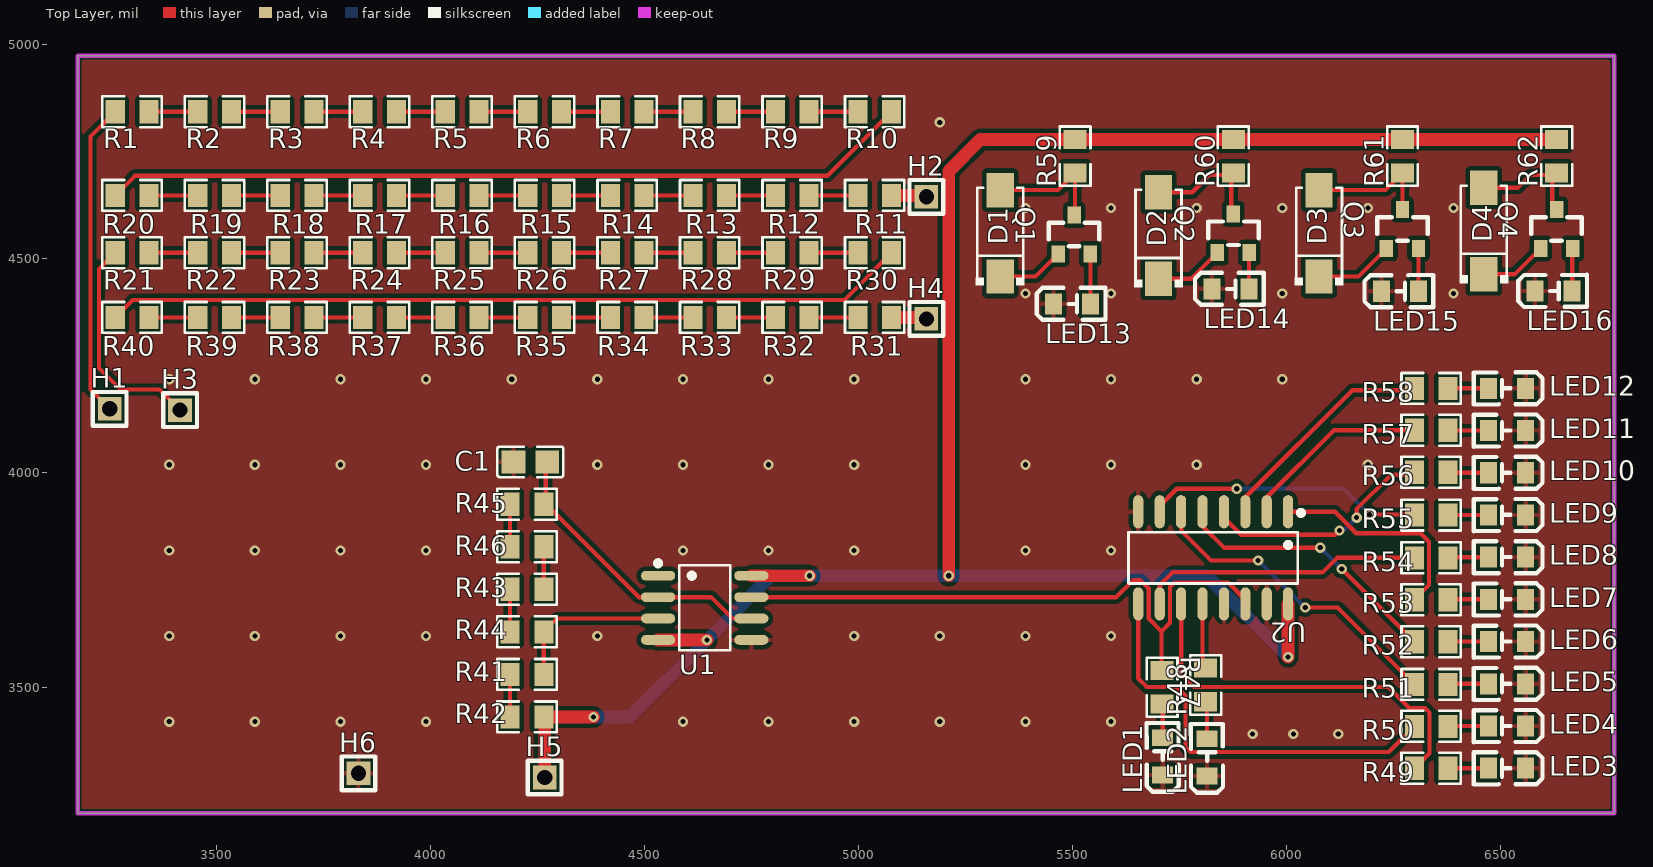
[diagram p0: Top Layer view]
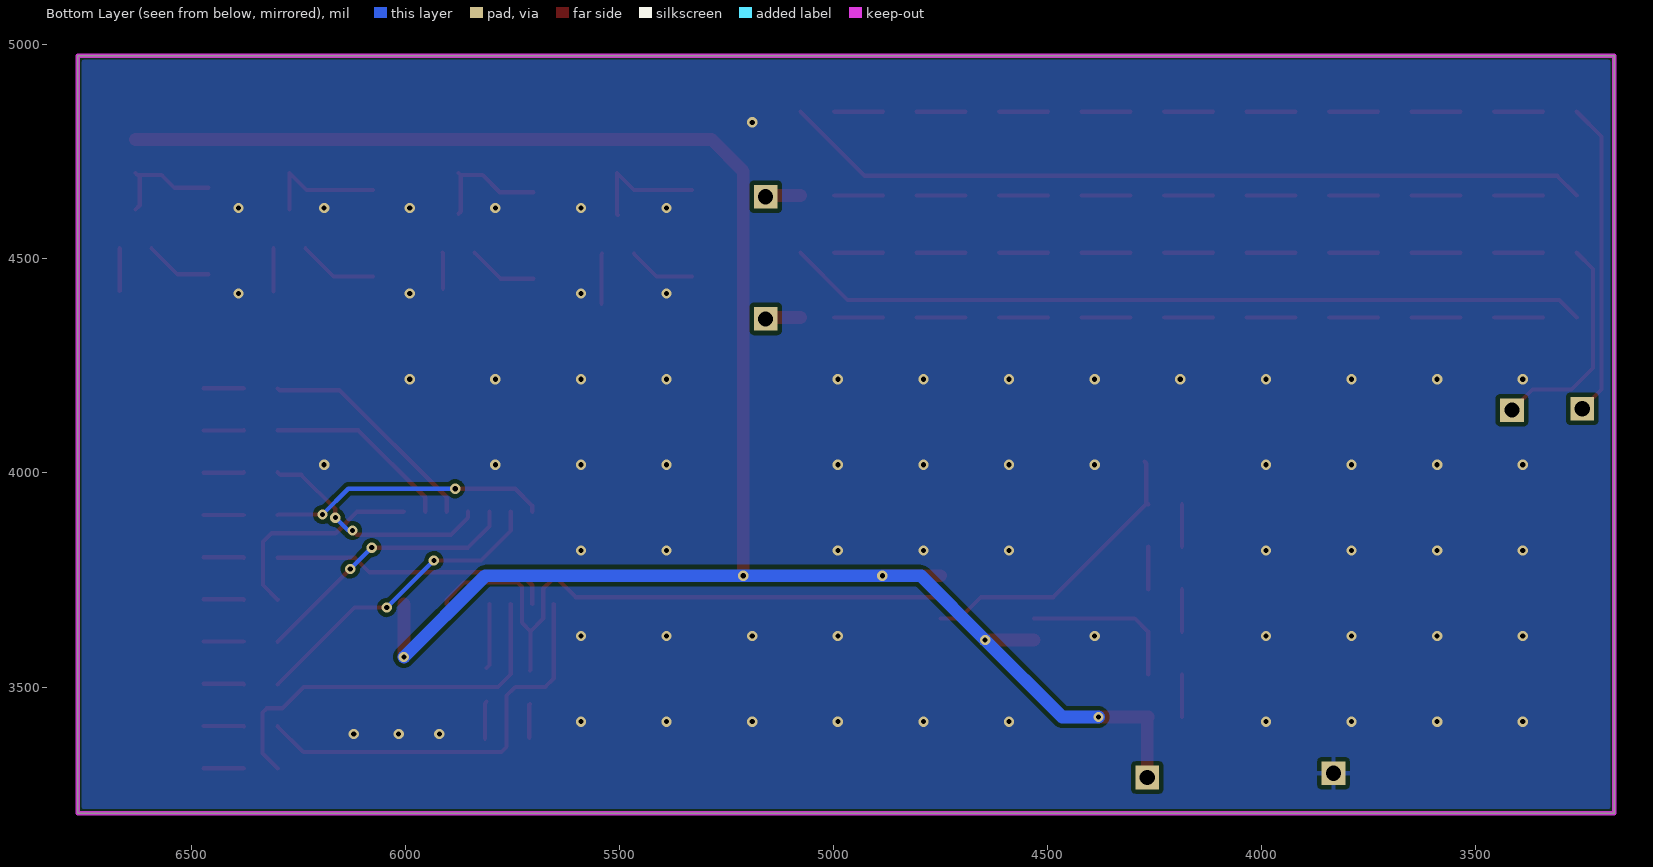
[diagram p1: Bottom Layer view, seen from below]
# Altium PCB MISC75384.pcbdoc
Units mil, origin at the board's own origin, x right, y up, seen from the top; angles counter-clockwise.
Board outline 3590 x 1770 mil, 2 copper layers (Top Layer, Bottom Layer), stack 62.206 mil thick; 95 components, 86 nets, 208 pads, 80 vias.

## Layer stack, top to bottom
Top Solder Mask Layer: solder mask 0.394, Dk 3.3
Top Layer: signal copper 1.379
Dielectric1: surface 59.449, FR4, Dk 4.5
Bottom Layer: signal copper 1.378
Bottom Solder Mask Layer: solder mask 0.394, Dk 3.3

## Board outline
3175,4975 3175,3205 6765,3205 6765,4975

## Design rules (kind name [scope] priority, off if disabled: settings)
BoardOutlineClearance copperThickness2oz_1 [All] p2 off: genericclearance=7.99 ignorepadtopadclearanceinfootprint=FALSE except(0: Arc-SplitContinuation Track-SplitContinuation SMDPad-SplitContinuation THPad-SplitContinuation Via-SplitContinuation Fill-SplitContinuation Region-SplitContinuation Poly-SplitContinuation Text-SplitContinuation Hole-SplitContinuation; 5.98: Arc-CutoutEdge SMDPad-CutoutEdge THPad-CutoutEdge Via-CutoutEdge Fill-CutoutEdge Region-CutoutEdge Text-CutoutEdge; 6.93: Hole-OutlineEdge Hole-CutoutEdge; 10: Poly-OutlineEdge Poly-CutoutEdge; 11.81: Arc-OutlineEdge Track-OutlineEdge SMDPad-OutlineEdge THPad-OutlineEdge Via-OutlineEdge Fill-OutlineEdge Region-OutlineEdge Text-OutlineEdge Track-CutoutEdge)
BoardOutlineClearance copperThickness1oz_1 [All] p4: genericclearance=4.02 ignorepadtopadclearanceinfootprint=FALSE except(0: Arc-SplitContinuation Track-SplitContinuation SMDPad-SplitContinuation THPad-SplitContinuation Via-SplitContinuation Fill-SplitContinuation Region-SplitContinuation Poly-SplitContinuation Text-SplitContinuation Hole-SplitContinuation; 6: SMDPad-CutoutEdge THPad-CutoutEdge Via-CutoutEdge Fill-CutoutEdge Region-CutoutEdge Text-CutoutEdge; 6.93: Hole-OutlineEdge Hole-CutoutEdge; 10: Poly-OutlineEdge Poly-CutoutEdge; 11.8: Arc-OutlineEdge Track-OutlineEdge SMDPad-OutlineEdge THPad-OutlineEdge Via-OutlineEdge Fill-OutlineEdge Region-OutlineEdge Text-OutlineEdge; 11.81: Arc-CutoutEdge Track-CutoutEdge)
Clearance copperThickness2oz [All] p1 off: gap=7.99 ignorepadtopadclearanceinfootprint=FALSE except(5.98: SMDPad-Track SMDPad-SMDPad THPad-Track SMDPad-THPad THPad-THPad Track-Via SMDPad-Via THPad-Via Via-Via Fill-Track Region-Track Fill-SMDPad Region-SMDPad Fill-THPad Region-THPad Fill-Via Region-Via Fill-Fill Fill-Region Region-Region Arc-Track Arc-SMDPad Arc-THPad Arc-Via Fill-Arc Region-Arc Arc-Arc Text-Track SMDPad-Text Text-THPad Text-Via Fill-Text Region-Text Arc-Text Text-Text; 6.93: Hole-Track Hole-SMDPad Hole-THPad Hole-Via Fill-Hole Region-Hole Hole-Arc Hole-Text; 10: Poly-Track Poly-SMDPad Poly-THPad Poly-Via Poly-Fill Poly-Region Poly-Poly Poly-Arc Poly-Text Poly-Hole)
Clearance copperThickness1oz [All] p3: gap=4.02 ignorepadtopadclearanceinfootprint=FALSE except(5.98: SMDPad-Track SMDPad-SMDPad THPad-Track SMDPad-THPad THPad-THPad Track-Via SMDPad-Via THPad-Via Via-Via Fill-Track Region-Track Fill-SMDPad Region-SMDPad Fill-THPad Region-THPad Fill-Via Region-Via Fill-Fill Fill-Region Region-Region; 6: Arc-Track Arc-SMDPad Arc-THPad Arc-Via Fill-Arc Region-Arc Arc-Arc Text-Track SMDPad-Text Text-THPad Text-Via Fill-Text Region-Text Arc-Text Text-Text; 6.93: Hole-Track Hole-SMDPad Hole-THPad Hole-Via Fill-Hole Region-Hole Hole-Arc Hole-Text; 10: Poly-Track Poly-SMDPad Poly-THPad Poly-Via Poly-Fill Poly-Region Poly-Poly Poly-Arc Poly-Text Poly-Hole)
Creepage creepage [All] p1: checkdistance=0 ignoreinternallayers=TRUE applytopolygonpour=TRUE
DiffPairsRouting differentialPair [All] p1: maxlimit=6 minlimit=6 mostfreqgap=6 toplayer_minwidth=5 toplayer_prefwidth=10 toplayer_maxwidth=100 toplayer_mingap=6 toplayer_prefgap=6 toplayer_maxgap=6 bottomlayer_minwidth=5 bottomlayer_prefwidth=10 bottomlayer_maxwidth=100 bottomlayer_mingap=6 bottomlayer_prefgap=6 bottomlayer_maxgap=6 maxuncoupledlength=10
HoleToHoleClearance otherClearance [All] p1: gap=11.81 allowstackedmicrovias=TRUE
Length netLength [All] p1: minlimit=0 maxlimit=0
MatchedLengths netLengthTolerance [All] p1: tolerance=1000
PasteMaskExpansion pasteMaskExpansion [All] p1: expansion=0
PlaneConnect innerPlane [All] p1: planeconnectstyle=Relief reliefexpansion=20 reliefentries=4 reliefconductorwidth=10 reliefairgap=10
PolygonConnect copperRegion [(InNet('GND') OR InNet('$1N69'))] p1: connectstyle=Relief reliefconductorwidth=10 reliefentries=4 polygonreliefangle="90 Angle" airgapwidth=10 via.connectstyle=Relief via.reliefconductorwidth=10 via.reliefentries=4 via.polygonreliefangle="90 Angle" via.airgapwidth=10
RoutingVias viaSize [All] p1: holewidth=12.01 width=24.02 viastyle="Through Hole" minholewidth=11.81 minwidth=19.68 maxholewidth=248.03 maxwidth=393.7
SolderMaskExpansion solderMaskExpansion [IsVia] p1: expansion=-1000 istentingtop=TRUE
SolderMaskExpansion solderMaskExpansion [All] p2: expansion=2 istentingtop=FALSE
Width copperThickness2oz_2 [All] p1 off: maxlimit=100 minlimit=8 preferedwidth=10
Width copperThickness1oz_2 [All] p2: maxlimit=100 minlimit=5 preferedwidth=10

## Components (designator, comment, footprint, x,y, rotation, side; value= is the part's Value field where it differs from the comment)
C1 "100nF" C0805 4232.64,4025.93 r0 top
D1 "" SMA_1N4007 5330,4560 r90 top
D2 "" SMA_1N4007 5700,4555 r90 top
D3 "" SMA_1N4007 6075,4560 r90 top
D4 "" SMA_1N4007 6460,4565 r90 top
H1 "" HDR-TH_1P-V-M_XKB_X4611WV-01I-C28D40 3250,4150 r0 top
H2 "" HDR-TH_1P-V-M_XKB_X4611WV-01I-C28D40 5157.69,4645.25 r0 top
H3 "" HDR-TH_1P-V-M_XKB_X4611WV-01I-C28D40 3414.27,4146.83 r0 top
H4 "" HDR-TH_1P-V-M_XKB_X4611WV-01I-C28D40 5157.69,4359.98 r0 top
H5 "" HDR-TH_1P-V-M_XKB_X4611WV-01I-C28D40 4266.12,3288.68 r0 top
H6 "" HDR-TH_1P-V-M_XKB_X4611WV-01I-C28D40 3831.12,3298.4 r0 top
LED1 "" LED_0805 5710,3340 r90 top
LED2 "" LED_0805 5813.62,3337.66 r90 top
LED3 "" LED_0805 6512.42,3310.52 r180 top
LED4 "" LED_0805 6512.42,3409.12 r180 top
LED5 "" LED_0805 6512.42,3507.72 r180 top
LED6 "" LED_0805 6512.42,3606.31 r180 top
LED7 "" LED_0805 6512.42,3704.91 r180 top
LED8 "" LED_0805 6512.42,3803.51 r180 top
LED9 "" LED_0805 6512.42,3902.11 r180 top
LED10 "" LED_0805 6512.42,4000.71 r180 top
LED11 "" LED_0805 6512.42,4099.3 r180 top
LED12 "" LED_0805 6512.42,4197.9 r180 top
LED13 "" LED_0805 5500,4395 r0 top
LED14 "" LED_0805 5870,4430 r0 top
LED15 "" LED_0805 6266.02,4424.29 r0 top
LED16 "" LED_0805 6625,4425 r0 top
Q1 "" S8050_SOT-23 5502.85,4557.14 r270 top
Q2 "" S8050_SOT-23 5875,4560 r270 top
Q3 "" S8050_SOT-23 6270,4570 r270 top
Q4 "" S8050_SOT-23 6630,4570 r270 top
R1 "10K" R0805 3302.34,4844.04 r0 top
R2 "10K" R0805 3495.07,4844.04 r0 top
R3 "10K" R0805 3687.81,4844.04 r0 top
R4 "10K" R0805 3880.54,4844.04 r0 top
R5 "10K" R0805 4073.28,4844.04 r0 top
R6 "10K" R0805 4266.01,4844.04 r0 top
R7 "10K" R0805 4458.75,4844.04 r0 top
R8 "10K" R0805 4651.48,4844.04 r0 top
R9 "10K" R0805 4844.22,4844.04 r0 top
R10 "10K" R0805 5036.95,4844.04 r0 top
R11 "10K" R0805 5036.95,4648.25 r180 top
R12 "10K" R0805 4844.22,4648.25 r180 top
R13 "10K" R0805 4651.48,4648.25 r180 top
R14 "10K" R0805 4458.75,4648.25 r180 top
R15 "10K" R0805 4266.01,4648.25 r180 top
R16 "10K" R0805 4073.28,4648.25 r180 top
R17 "10K" R0805 3880.54,4648.25 r180 top
R18 "10K" R0805 3687.81,4648.25 r180 top
R19 "10K" R0805 3495.07,4648.25 r180 top
R20 "10K" R0805 3302.34,4648.25 r180 top
R21 "15K" R0805 3302.34,4514.29 r0 top
R22 "15K" R0805 3495.07,4514.29 r0 top
R23 "15K" R0805 3687.81,4514.29 r0 top
R24 "15K" R0805 3880.54,4514.29 r0 top
R25 "15K" R0805 4073.28,4514.29 r0 top
R26 "15K" R0805 4266.01,4514.29 r0 top
R27 "15K" R0805 4458.75,4514.29 r0 top
R28 "15K" R0805 4651.48,4514.29 r0 top
R29 "15K" R0805 4844.22,4514.29 r0 top
R30 "15K" R0805 5036.95,4514.29 r0 top
R31 "15K" R0805 5036.95,4363.3 r180 top
R32 "15K" R0805 4844.22,4363.3 r180 top
R33 "15K" R0805 4651.48,4363.3 r180 top
R34 "15K" R0805 4458.75,4363.3 r180 top
R35 "15K" R0805 4266.01,4363.3 r180 top
R36 "15K" R0805 4073.28,4363.3 r180 top
R37 "15K" R0805 3880.54,4363.3 r180 top
R38 "15K" R0805 3687.81,4363.3 r180 top
R39 "15K" R0805 3495.07,4363.3 r180 top
R40 "15K" R0805 3302.34,4363.3 r180 top
R41 "10K" R0805 4224.66,3529.41 r0 top
R42 "10K" R0805 4224.66,3430 r180 top
R43 "10K" R0805 4224.66,3728.23 r0 top
R44 "10K" R0805 4224.66,3628.82 r180 top
R45 "10K" R0805 4224.66,3927.05 r0 top
R46 "10K" R0805 4224.66,3827.64 r180 top
R47 "1K" R0805 5708.24,3499.45 r270 top
R48 "1K" R0805 5810,3505 r90 top
R49 "10K" R0805 6337.09,3310.12 r0 top
R50 "10K" R0805 6337.09,3408.02 r0 top
R51 "10K" R0805 6337.09,3505.92 r0 top
R52 "10K" R0805 6337.09,3605.92 r0 top
R53 "10K" R0805 6337.09,3703.82 r0 top
R54 "10K" R0805 6337.09,3801.71 r0 top
R55 "10K" R0805 6337.09,3901.71 r0 top
R56 "10K" R0805 6337.09,4001.71 r0 top
R57 "10K" R0805 6337.09,4099.61 r0 top
R58 "10K" R0805 6337.09,4197.51 r0 top
R59 "1K" R0805 5505,4740 r90 top
R60 "1K" R0805 5875,4740 r90 top
R61 "1K" R0805 6270,4740 r90 top
R62 "1K" R0805 6630,4740 r90 top
U1 "NE555" SOP-8_L5.0-W4.0-P1.27-LS6.0-BL 4640,3685 r270 top
U2 "CD4017BM96G4" SOIC-16_L9.9-W3.9-P1.27-LS6.0-BL 5827.85,3801.71 r180 top

## Footprints (in the part's own frame and the unit in brackets; to place one, negate y for a bottom-side part, rotate by r counter-clockwise, add the part's x,y. Pads: shape width x height; smd on the part's side, far side on the other; paste and mask are expansions set on the pad)
C0805 [mm]
  rect 1.41x1.35 smd paste-100 mask+0.051: 1(-1,0) 2(1,0)
  silkscreen extent -1.96,-0.9 1.96,0.9
HDR-TH_1P-V-M_XKB_X4611WV-01I-C28D40 [mm]
  rect 1.4x1.4 hole 0.9: 1(0,0)
  silkscreen extent -1,-1 1,1
LED_0805 [mm]
  rect 1x1.25 smd paste+0 mask+0.051: 1(-1.15,0.005) 2(1.05,0.005)
  silkscreen extent -2.15,-0.94 1.93,0.97
R0805 [mm]
  rect 1.133x1.377 smd paste-100 mask+0.051: 1(-1,0) 2(1,0)
  silkscreen extent -1.76,-0.92 1.76,0.92
S8050_SOT-23 [mm]
  rect 1x0.8 smd paste+0 mask+0.051: 1(1.15,-0.95) 2(1.15,0.95) 3(-1.15,0)
  silkscreen extent -0.7,-1.5 0.7,1.5
SMA_1N4007 [mil]
  rect 80.57x63.78 smd paste+0 mask+2: 1(-101,0) 2(101,0)
  silkscreen extent -121,-57 106,57
SOIC-16_L9.9-W3.9-P1.27-LS6.0-BL [mil]
  oval 23.7x77.6 smd: 1(-175,-107.7) 2(-125,-107.7) 3(-75,-107.7) 4(-25,-107.7) 5(25,-107.7) 6(75,-107.7) 7(125,-107.7) 8(175,-107.7) 9(175,107.7) 10(125,107.7) 11(75,107.7) 12(25,107.7) 13(-25,107.7) 14(-75,107.7) 15(-125,107.7) 16(-175,107.7)
  silkscreen extent -211,-111 198,60
SOP-8_L5.0-W4.0-P1.27-LS6.0-BL [mil]
  oval 22.6x80.14 smd: 1(-75,-108.97) 2(-25,-108.97) 3(25,-108.97) 4(75,-108.97) 5(75,108.97) 6(25,108.97) 7(-25,108.97) 8(-75,108.97)
  silkscreen extent -110,-115 99,60

## Via types
v1: diameter 24.02, hole 12, Top Layer to Bottom Layer, 80 vias

## Nets (pads, with @x,y where several pads share a name; then routed paths per layer and width w, separated by ;. In a path a pad name is that pad's centre, name@x,y a point inside that pad or via, vN(x,y) a via of type N, cw(c..) or ccw(c..) an arc to the next point about the centre after c; other vN are vias at no path point)
$1N1: R1.2 R2.1 | length 114
  Top Layer w10: R1.2 R2.1
$1N2: R2.2 R3.1 | length 114
  Top Layer w10: R2.2 R3.1
$1N3: R3.2 R4.1 | length 114
  Top Layer w10: R3.2 R4.1
$1N4: R4.2 R5.1 | length 114
  Top Layer w10: R4.2 R5.1
$1N5: R5.2 R6.1 | length 114
  Top Layer w10: R5.2 R6.1
$1N6: R7.2 R8.1 | length 114
  Top Layer w10: R7.2 R8.1
$1N7: R6.2 R7.1 | length 114
  Top Layer w10: R6.2 R7.1
$1N8: R9.2 R10.1 | length 114
  Top Layer w10: R9.2 R10.1
$1N9: R8.2 R9.1 | length 114
  Top Layer w10: R8.2 R9.1
$1N10: R18.2 R19.1 | length 114
  Top Layer w10: R19.1 R18.2
$1N11: R16.2 R17.1 | length 114
  Top Layer w10: R17.1 R16.2
$1N12: R17.2 R18.1 | length 114
  Top Layer w10: R18.1 R17.2
$1N13: R19.2 R20.1 | length 114
  Top Layer w10: R20.1 R19.2
$1N14: R15.2 R16.1 | length 114
  Top Layer w10: R16.1 R15.2
$1N15: R14.2 R15.1 | length 114
  Top Layer w10: R15.1 R14.2
$1N16: R13.2 R14.1 | length 114
  Top Layer w10: R14.1 R13.2
$1N17: R12.2 R13.1 | length 114
  Top Layer w10: R13.1 R12.2
$1N18: R11.2 R12.1 | length 114
  Top Layer w10: R12.1 R11.2
$1N19: R10.2 R20.2 | length 1894.5
  Top Layer w10: R20.2 3308.76,4694.04 4926.32,4694.04 R10.2
$1N24: R30.2 R40.2 | length 1875.9
  Top Layer w10: R40.2 3303.96,4404.3 4966.32,4404.3 R30.2
$1N25: R28.2 R29.1 | length 114
  Top Layer w10: R28.2 R29.1
$1N26: R38.2 R39.1 | length 114
  Top Layer w10: R39.1 R38.2
$1N27: R26.2 R27.1 | length 114
  Top Layer w10: R26.2 R27.1
$1N28: R36.2 R37.1 | length 114
  Top Layer w10: R37.1 R36.2
$1N29: R27.2 R28.1 | length 114
  Top Layer w10: R27.2 R28.1
$1N30: R39.2 R40.1 | length 114
  Top Layer w10: R40.1 R39.2
$1N31: R29.2 R30.1 | length 114
  Top Layer w10: R29.2 R30.1
$1N32: R37.2 R38.1 | length 114
  Top Layer w10: R38.1 R37.2
$1N33: R25.2 R26.1 | length 114
  Top Layer w10: R25.2 R26.1
$1N34: R35.2 R36.1 | length 114
  Top Layer w10: R36.1 R35.2
$1N35: R24.2 R25.1 | length 114
  Top Layer w10: R24.2 R25.1
$1N36: R34.2 R35.1 | length 114
  Top Layer w10: R35.1 R34.2
$1N37: R23.2 R24.1 | length 114
  Top Layer w10: R23.2 R24.1
$1N38: R33.2 R34.1 | length 114
  Top Layer w10: R34.1 R33.2
$1N39: R22.2 R23.1 | length 114
  Top Layer w10: R22.2 R23.1
$1N40: R32.2 R33.1 | length 114
  Top Layer w10: R33.1 R32.2
$1N41: R21.2 R22.1 | length 114
  Top Layer w10: R21.2 R22.1
$1N42: R31.2 R32.1 | length 114
  Top Layer w10: R32.1 R31.2
$1N44: R41.2 R44.1 U1.3 | length 379.3
  Top Layer w10: R41.2 R44.1 4295.21,3660 U1.3
$1N45: R41.1 R42.2 | length 99.4
  Top Layer w10: R42.2 R41.1
$1N47: R43.1 R44.2 | length 99.4
  Top Layer w10: R44.2 R43.1
$1N48: R45.1 R46.2 | length 99.4
  Top Layer w10: R46.2 R45.1
$1N49: R43.2 R46.1 | length 99.4
  Top Layer w10: R43.2 R46.1
$1N56: LED1.2 R47.2 | length 79.4
  Top Layer w10: R47.2 5709.79,3458.52 LED1.2
$1N63: R48.2 U2.12 | length 152.6
  Top Layer w10: U2.12 5802.85,3551.51 R48.2
$1N64: LED2.2 R48.1 | length 88
  Top Layer w10: R48.1 5813.42,3462.21 LED2.2
$1N66: R49.1 U2.11 | length 925.7
  Top Layer w10: U2.11 5752.85,3530.21 5782.85,3500.21 6236.55,3500.21 6286.55,3450.21 6322.85,3450.21 6332.85,3440.21 6332.85,3345.26 R49.1
$1N67: LED3.2 R49.2 | length 94.4
  Top Layer w10: R49.2@6376.65,3310.31 LED3.2
$1N68: R50.1 U2.9 | length 985.1
  Top Layer w10: U2.9 5652.85,3520.21 5672.85,3500.21 5742.85,3500.21 5762.85,3480.21 5762.85,3360.21 5775.04,3348.02 6237.72,3348.02 R50.1
$1N69: R51.1 U2.6 | length 737.7
  Top Layer w10: U2.6 5752.85,3865.61 5822.85,3795.61 v1(5932.85,3795.61) ; v1(6042.85,3685.61) 6118.03,3685.61 R51.1
  Bottom Layer w10: v1(5932.85,3795.61) v1(6042.85,3685.61)
$1N70: R52.1 U2.5 | length 640.4
  Top Layer w10: U2.5 5802.85,3875.61 5852.85,3825.61 v1(6078.03,3825.61) ; v1(6128.03,3775.61) R52.1
  Bottom Layer w10: v1(6078.03,3825.61) v1(6128.03,3775.61)
$1N71: R53.1 U2.1 | length 508.1
  Top Layer w10: U2.1 6112.12,3909.41 6162.12,3859.41 6312.12,3859.41 6332.12,3839.41 6332.12,3738.22 R53.1
$1N72: R54.1 U2.10 | length 665.1
  Top Layer w10: U2.10 5702.85,3737.81 5732.85,3767.81 6082.85,3767.81 6116.75,3801.71 R54.1
$1N73: R55.1 U2.7 | length 650.7
  Top Layer w10: U2.7 5702.85,3923.21 5742.85,3963.21 v1(5882.85,3963.21) ; v1(6192.85,3903.21) 6296.22,3903.21 R55.1
  Bottom Layer w10: v1(5882.85,3963.21) 6132.85,3963.21 v1(6192.85,3903.21)
$1N74: R56.1 U2.4 | length 547.5
  Top Layer w10: U2.4 5852.85,3895.61 5892.85,3855.61 6112.85,3855.61 v1(6122.85,3865.61) ; v1(6162.85,3895.61) 6162.85,3915.61 6242.85,3995.61 6291.62,3995.61 R56.1
  Bottom Layer w10: v1(6122.85,3865.61) 6132.85,3865.61 v1(6162.85,3895.61)
$1N75: R57.1 U2.2 | length 443.4
  Top Layer w10: U2.2 5952.85,3943.21 6109.25,4099.61 R57.1
$1N76: R58.1 U2.3 | length 534
  Top Layer w10: U2.3 5902.85,3943.21 6152.85,4193.21 6293.42,4193.21 R58.1
$1N77: LED4.2 R50.2 | length 95
  Top Layer w10: R50.2 6377.35,3408.91 LED4.2
$1N78: LED5.2 R51.2 | length 95.3
  Top Layer w10: R51.2 6378.05,3507.51 LED5.2
$1N79: LED6.2 R52.2 | length 94.4
  Top Layer w10: R52.2@6376.65,3606.11 LED6.2
$1N80: LED7.2 R53.2 | length 95
  Top Layer w10: R53.2 6377.35,3704.71 LED7.2
$1N81: LED8.2 R54.2 | length 95.3
  Top Layer w10: R54.2 6378.05,3803.31 LED8.2
$1N82: LED9.2 R55.2 | length 94.4
  Top Layer w10: R55.2@6376.65,3901.9 LED9.2
$1N83: LED10.2 R56.2 | length 95.1
  Top Layer w10: R56.2 6377.67,4000.5 LED10.2
$1N84: LED11.2 R57.2 | length 94.8
  Top Layer w10: R57.2 6376.97,4099.1 LED11.2
$1N85: LED12.2 R58.2 | length 94.4
  Top Layer w10: R58.2@6376.65,4197.7 LED12.2
$1N87: D1.2 Q1.3 R59.1 | length 290.5
  Top Layer w10: D1.2 5465.37,4661 R59.1 5505,4604.56 Q1.3
$1N88: D1.1 Q1.1 | length 157.3
  Top Layer w10: D1.1 5412.59,4459 Q1.1
$1N89: LED13.2 Q1.2 | length 117.1
  Top Layer w10: Q1.2 5541.34,4510.78 LED13.2
$1N94: LED14.2 Q2.2 | length 85
  Top Layer w10: LED14.2 5911.34,4513.66 Q2.2
$1N95: D2.1 Q2.1 | length 162.8
  Top Layer w10: D2.1 5776.87,4454 Q2.1
$1N96: D2.2 Q2.3 R60.1 | length 286.2
  Top Layer w10: D2.2 5778.74,4656 5818.74,4696 R60.1@5870,4696 ; Q2.3 5870,4610.28 R60.1@5870,4696 ; R60.1 R60.1@5870,4696
$1N101: LED15.2 Q3.2 | length 100.2
  Top Layer w10: LED15.2 Q3.2
$1N102: LED16.2 Q4.2 | length 100
  Top Layer w10: LED16.2 6666.34,4523.66 Q4.2
$1N103: D3.1 Q3.1 | length 184.8
  Top Layer w10: D3.1 6166.88,4459 Q3.1
$1N104: D4.1 Q4.1 | length 157.8
  Top Layer w10: D4.1 6531.88,4464 Q4.1
$1N105: D3.2 Q3.3 R61.1 | length 296.8
  Top Layer w10: D3.2 6230.37,4661 R61.1 Q3.3
$1N106: D4.2 Q4.3 R62.1 | length 269.2
  Top Layer w10: D4.2 6538.74,4666 6568.74,4696 R62.1@6620,4696 ; Q4.3 6620,4625.28 R62.1@6620,4696 ; R62.1 6625.37,4696 R62.1@6620,4696
+5V: H5.1 R42.1 R59.2 R60.2 R61.2 R62.2 U1.4 U1.8 U2.16 | length 4866.2
  Top Layer w30: H5.1 4266.12,3427.91 R42.1 v1(4380,3430) ; U1.4 v1(4645,3610) ; U1.8 v1(4885,3760) ; v1(5210,3760) 5210,4705 5284.37,4779.37 R59.2 R60.2 R61.2 R62.2 ; v1(6002.85,3570) U2.16
  Bottom Layer w30: v1(4380,3430) 4465,3430 v1(4645,3610) 4795,3760 v1(4885,3760) v1(5210,3760) 5812.85,3760 v1(6002.85,3570)
GND: C1.1 H6.1 LED1.1 LED2.1 LED3.1 LED4.1 LED5.1 LED6.1 LED7.1 LED8.1 LED9.1 LED10.1 LED11.1 LED12.1 LED13.1 LED14.1 LED15.1 LED16.1 U1.5 U2.8 U2.13 U2.15
  other v1: 5920,3390 6015,3390 6120,3390 3389.1,3419.1 3589.1,3419.1 3789.1,3419.1 3989.1,3419.1 4589.1,3419.1 4789.1,3419.1 4989.1,3419.1 5189.1,3419.1 5389.1,3419.1 5589.1,3419.1 3389.1,3619.1 3589.1,3619.1 3789.1,3619.1 3989.1,3619.1 4389.1,3619.1 4989.1,3619.1 5189.1,3619.1 5389.1,3619.1 5589.1,3619.1 3389.1,3819.1 3589.1,3819.1 3789.1,3819.1 3989.1,3819.1 4589.1,3819.1 4789.1,3819.1 4989.1,3819.1 5389.1,3819.1 5589.1,3819.1 3389.1,4019.1 3589.1,4019.1 3789.1,4019.1 3989.1,4019.1 4389.1,4019.1 4589.1,4019.1 4789.1,4019.1 4989.1,4019.1 5389.1,4019.1 5589.1,4019.1 5789.1,4019.1 6189.1,4019.1 3389.1,4219.1 3589.1,4219.1 3789.1,4219.1 3989.1,4219.1 4189.1,4219.1 4389.1,4219.1 4589.1,4219.1 4789.1,4219.1 4989.1,4219.1 5389.1,4219.1 5589.1,4219.1 5789.1,4219.1 5989.1,4219.1 5389.1,4419.1 5589.1,4419.1 5989.1,4419.1 6389.1,4419.1 5389.1,4619.1 5589.1,4619.1 5789.1,4619.1 5989.1,4619.1 6189.1,4619.1 6389.1,4619.1 5189.1,4819.1
R0805IN: H3.1 R21.1 | length 515
  Top Layer w10: R21.1 3225,4476.33 3225,4245 3275,4195 3366.1,4195 H3.1
R0805OUT: H4.1 R31.1 | length 82.7
  Top Layer w30: R31.1 5154.37,4363.3 H4.1
RAIN: H1.1 R1.1 | length 736.7
  Top Layer w10: H1.1 3205,4195 3205,4786.08 R1.1
RAOUT: H2.1 R11.1 | length 82.6
  Top Layer w30: R11.1 5154.7,4648.25 H2.1
THR: C1.2 R45.2 U1.2 U1.6 | length 695.7
  Top Layer w10: R45.2 R45.2@4268.91,3927.05 ; C1.2 4268.91,4022.84 R45.2@4268.91,3927.05 ; U1.6 4704.84,3660 4654.84,3710 U1.2 4485.96,3710 R45.2@4268.91,3927.05
VO: R47.1 U1.7 U2.14 | length 1475.8
  Top Layer w10: U1.7 5601.52,3710 5641.52,3750 5657.06,3750 5677.06,3730 5677.06,3660 5707.06,3630 ; R47.1 5707.06,3540 5707.06,3630 ; U2.14 5902.85,3704.01 5862.85,3744.01 5737.06,3744.01 5727.06,3734.01 5727.06,3650 5707.06,3630
pads on no net: U1.1

## Polygon pours and split planes (outlines as drawn)
GND on Top Layer (solid, remove dead copper, pour order 0): 3000,5205 3000,3010 7135,3010 7135,5205
GND on Bottom Layer (solid, remove dead copper, pour order 2): 3060,5075 3060,3000 6870,3000 6870,5075

## Keep-outs
Board Outline Layer:
  the board outline again, w10